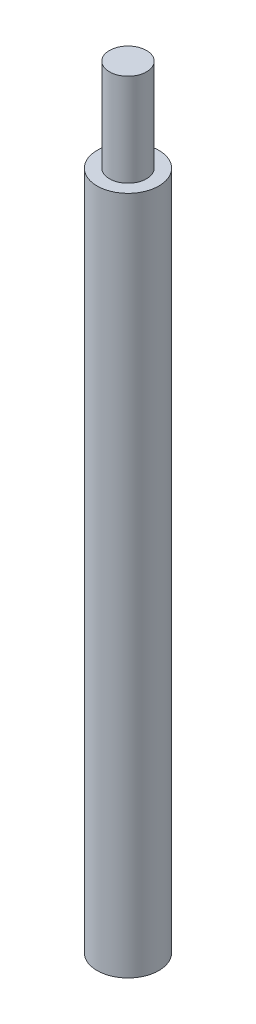
SolidWorks part; units mm, degrees
ref_plane "Front Plane" through (0, 0, 0) normal (0, 0, 1) x (1, 0, 0)
ref_plane "Top Plane" through (0, 0, 0) normal (0, 1, 0) x (1, 0, 0)
ref_plane "Right Plane" through (0, 0, 0) normal (1, 0, 0) x (0, 0, -1)
sketch "Sketch1" plane through (0, 0, 0) normal (0, 1, 0) x (1, 0, 0)
  circle A0 centre (0, 0) radius 10
  dimension "D1" = 20
extrude "Boss-Extrude1" add sketch "Sketch1" along normal blind 250
sketch "Sketch2" plane through (0, 250, 0) normal (0, 1, 0) x (1, 0, 0)
  circle A0 centre (0, 0) radius 6
  dimension "D1" = 12
extrude "Cut-Extrude1" cut sketch "Sketch2" against normal blind 30 flip side to cut
